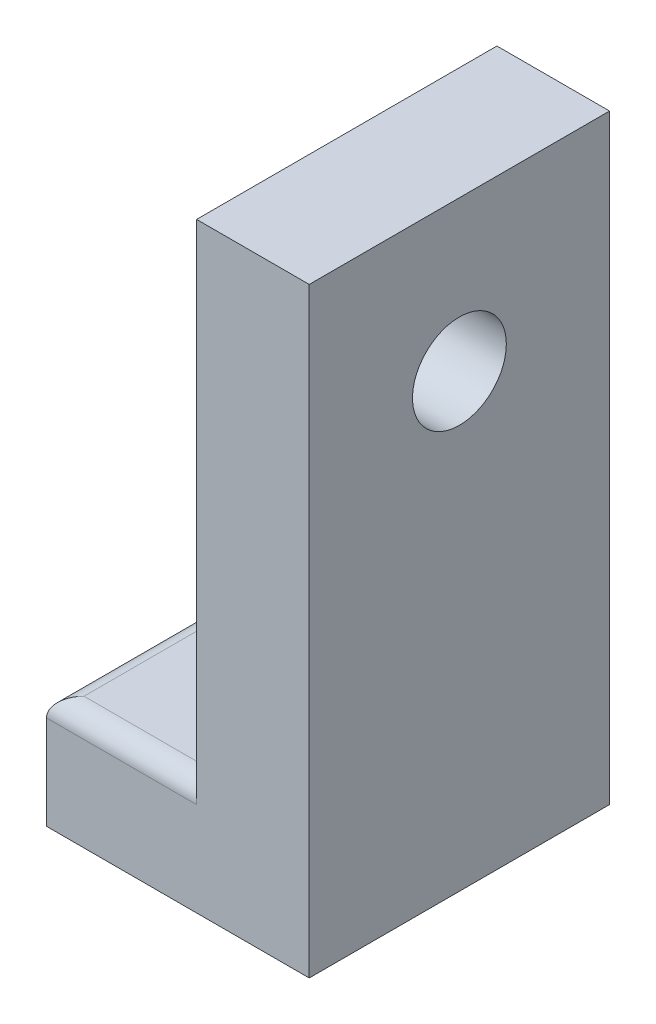
from build123d import *

# Parameters (mm, degrees)
EXTRUDE_1_DEPTH    = 8
HOLE_WIZARD_M3_1_D = 2.5
FILLET_1_R         = 0.5


with BuildPart() as part:
    # 草图1 → 凸台-拉伸1 (new body)
    with BuildSketch(Plane.XY):
        Polygon((-4, -16), (3, -16), (3, 0), (0, 0), (0, -13), (-4, -13), align=None)
    extrude(amount=EXTRUDE_1_DEPTH)

    # M3 螺纹孔1 (through all)
    with Locations(Plane(origin=(3, 0, 0), x_dir=(0, 0, -1), z_dir=(1, 0, 0))):
        with Locations((-4, -4)):
            Hole(HOLE_WIZARD_M3_1_D / 2)

    # 圆角1
    fillet_1_edges = [part.edges().sort_by_distance(p)[0] for p in [
        (-4, -13, 4),
        (-2, -13, 8),
        (-2, -13, 0),
    ]]
    fillet(fillet_1_edges, radius=FILLET_1_R)


solid = part.part
